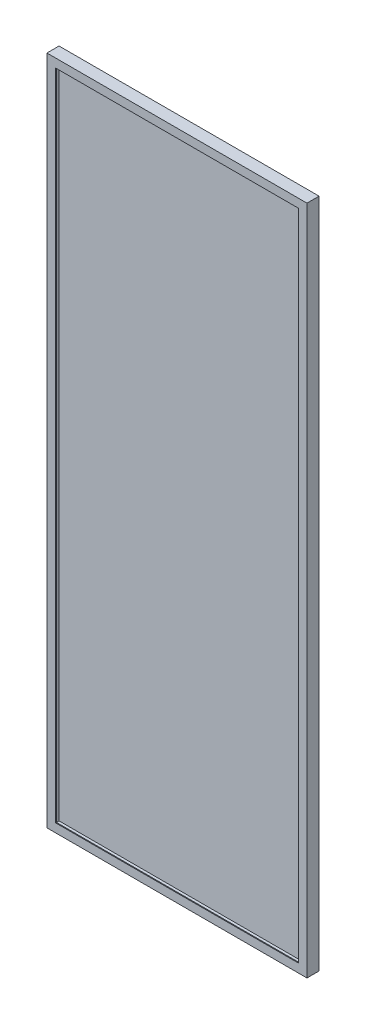
from build123d import *

# Parameters (mm, degrees)
SKETCH_1_W      = 601
SKETCH_1_H      = 1551
EXTRUDE_1_DEPTH = 28
SHELL_1_T       = -2
SKETCH_2_W      = 601
SKETCH_2_H      = 1551
SKETCH_2_W_2    = 561
SKETCH_2_H_2    = 1511
EXTRUDE_2_DEPTH = 2


with BuildPart() as part:
    # 草图1 → 凸台-拉伸1 (new body)
    with BuildSketch(Plane.XY):
        with Locations((300.5, 775.5)):
            Rectangle(SKETCH_1_W, SKETCH_1_H)
    extrude(amount=EXTRUDE_1_DEPTH)

    # 抽壳1
    shell_1_openings = [part.faces().sort_by_distance(p)[0] for p in [
        (300.5, 775.5, 28),
    ]]
    offset(amount=SHELL_1_T, openings=shell_1_openings, kind=Kind.INTERSECTION)

    # 草图2 → 凸台-拉伸2 (add)
    with BuildSketch(Plane.XY.offset(28)):
        with Locations((300.5, 775.5)):
            Rectangle(SKETCH_2_W, SKETCH_2_H)
        with Locations((300.5, 775.5)):
            Rectangle(SKETCH_2_W_2, SKETCH_2_H_2, mode=Mode.SUBTRACT)
    extrude(amount=-EXTRUDE_2_DEPTH)


solid = part.part
